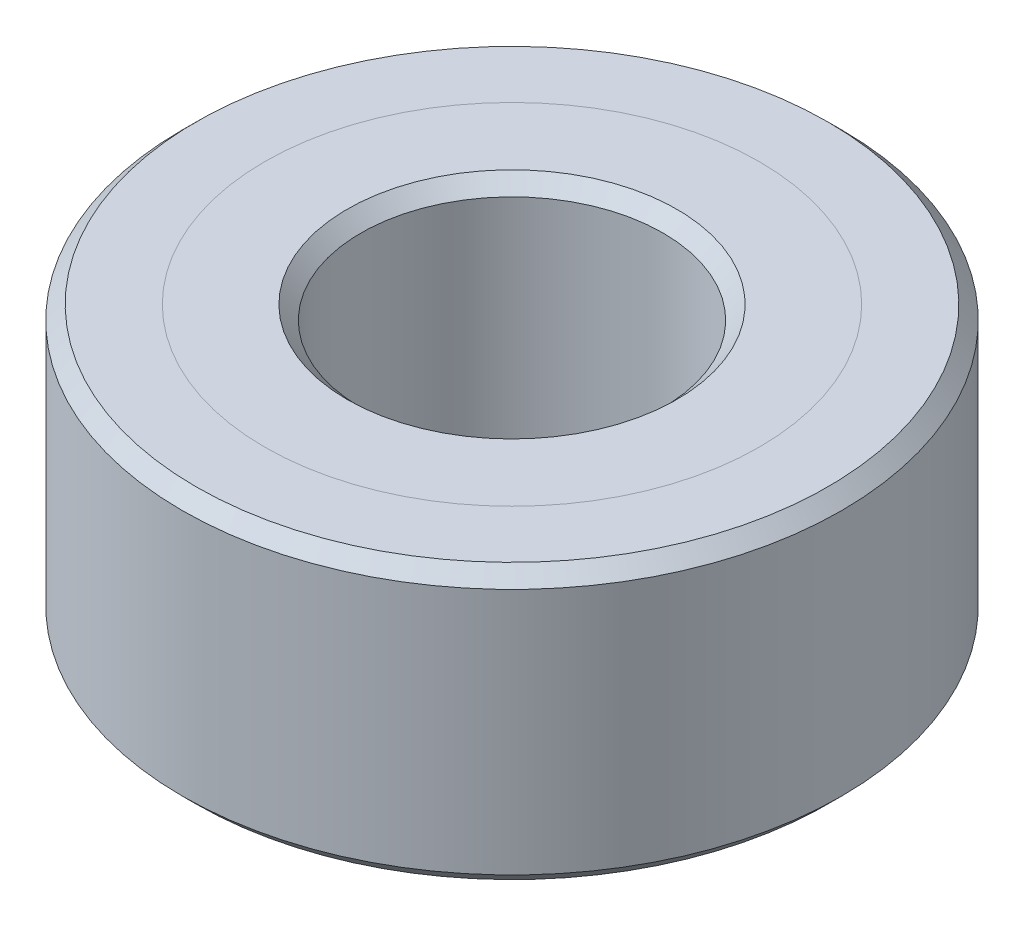
from build123d import *

# Parameters (mm, degrees)
SKETCH1_R           = 15
SKETCH1_R_2         = 5.5
BOSS_EXTRUDE1_DEPTH = 10
CHAMFER1_SIZE       = 0.5
CUT_EXTRUDE1_START  = -10
SKETCH2_R           = 15
SKETCH2_R_2         = 9
CUT_EXTRUDE1_DEPTH  = 10
SKETCH3_R           = 12
SKETCH3_R_2         = 9
BOSS_EXTRUDE2_DEPTH = 10
CHAMFER2_SIZE       = 0.5
CHAMFER3_SIZE       = 0.5


with BuildPart() as part:
    # Sketch1 → Boss-Extrude1 (new body)
    with BuildSketch(Plane(origin=(0, 0, 0), x_dir=(1, 0, 0), z_dir=(0, 1, 0))):
        with Locations(Location((0, 0, 0), (0, 0, 270))):
            Circle(SKETCH1_R)
        with Locations(Location((0, 0, 0), (0, 0, 270))):
            Circle(SKETCH1_R_2, mode=Mode.SUBTRACT)
    extrude(amount=BOSS_EXTRUDE1_DEPTH)

    # Chamfer1
    chamfer1_edges = [part.edges().sort_by_distance(p)[0] for p in [
        (0, 0, -15),
        (0, 10, -15),
    ]]
    chamfer(chamfer1_edges, length=CHAMFER1_SIZE)

    # Sketch2 → Cut-Extrude1 (cut)
    with BuildSketch(Plane(origin=(0, 10, 0), x_dir=(1, 0, 0), z_dir=(0, 1, 0)).offset(CUT_EXTRUDE1_START)):
        Circle(SKETCH2_R)
        with Locations(Location((0, 0, 0), (0, 0, 270))):
            Circle(SKETCH2_R_2, mode=Mode.SUBTRACT)
    extrude(amount=CUT_EXTRUDE1_DEPTH, mode=Mode.SUBTRACT)

    # Chamfer3
    chamfer3_edges = [part.edges().sort_by_distance(p)[0] for p in [
        (0, 0, -5.5),
        (0, 10, -5.5),
    ]]
    chamfer(chamfer3_edges, length=CHAMFER3_SIZE)


with BuildPart() as body_2:
    # Sketch3 → Boss-Extrude2 (new body)
    with BuildSketch(Plane(origin=(0, 10, 0), x_dir=(1, 0, 0), z_dir=(0, 1, 0))):
        with Locations(Location((0, 0, 0), (0, 0, 270))):
            Circle(SKETCH3_R)
        with Locations(Location((0, 0, 0), (0, 0, 270))):
            Circle(SKETCH3_R_2, mode=Mode.SUBTRACT)
    extrude(amount=-BOSS_EXTRUDE2_DEPTH)

    # Chamfer2
    chamfer2_edges = [body_2.edges().sort_by_distance(p)[0] for p in [
        (0, 10, -12),
        (0, 0, -12),
    ]]
    chamfer(chamfer2_edges, length=CHAMFER2_SIZE)


solid = Compound([part.part, body_2.part])
